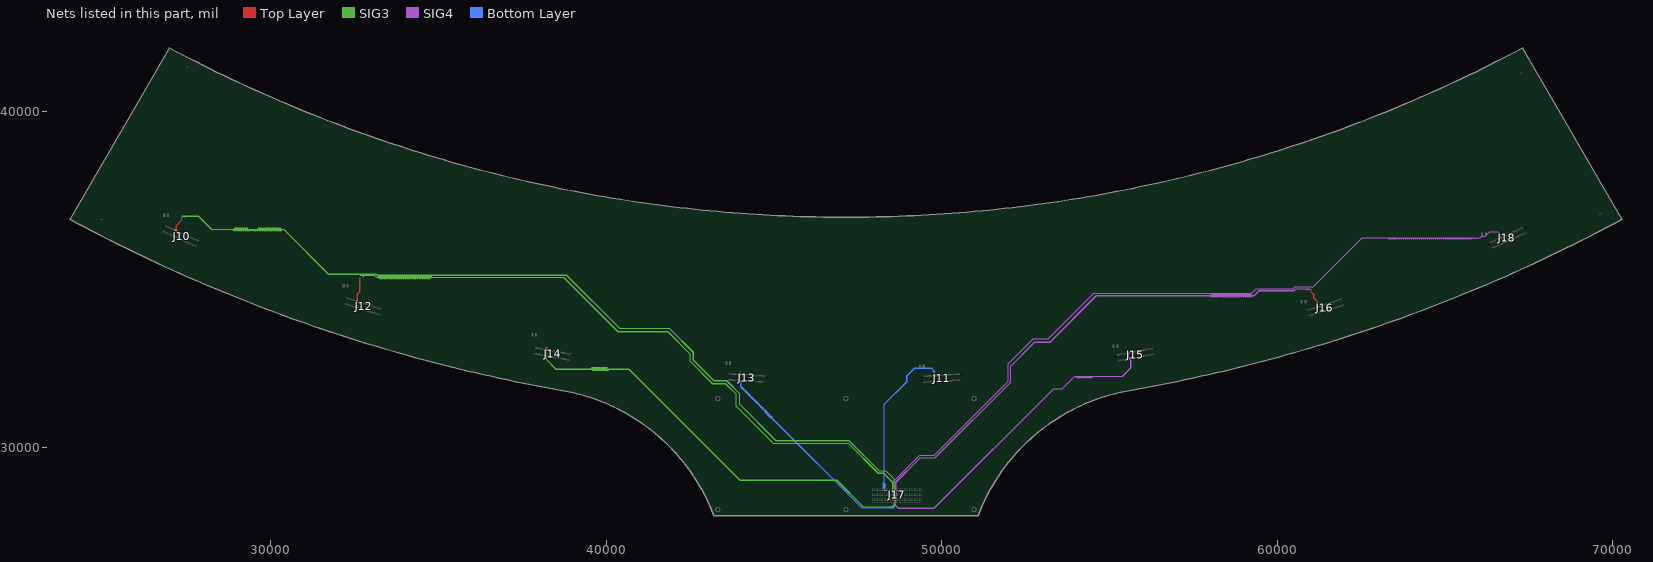
[diagram p0: the nets of this part, all layers, seen from the top]
# Altium PCB MISC86329.PcbDoc (part 6 of 11)
Units mil, origin at the board's own origin, x right, y up, seen from the top; angles counter-clockwise.
Board outline 46247.15 x 13937.21 mil, 6 copper layers (Top Layer, GND2, SIG3, SIG4, POWER5, Bottom Layer); 17 components, 210 nets, 908 pads, 1109 vias.

## Via types
v1: diameter 24, hole 12, Top Layer to Bottom Layer, 684 vias
v2: diameter 18, hole 9, Top Layer to Bottom Layer, 425 vias

## Nets (pads, with @x,y where several pads share a name; then routed paths per layer and width w, separated by ;. In a path a pad name is that pad's centre, name@x,y a point inside that pad or via, vN(x,y) a via of type N, cw(c..) or ccw(c..) an arc to the next point about the centre after c; other vN are vias at no path point) (continued)
DATAIN4N_CH0: J10.24 J17.G17 | length 28226.9
  Top Layer w5: J10.24@27193.09,36458.02 27193.09,36485.62 27204,36496.53 27204,36609 27363,36768 27363,36860.5 v2(27369.5,36867) ; v2(48564.09,28692.61) J17.G17@48587.89,28668.8
  SIG3 w5: v2(27369.5,36867) 27363,36873.5 27363,36882.86 27377.14,36897 27429,36897 27434,36892 27434,36882.36 27439,36877.36 27449,36877.36 27454,36882.36 27454,36892 27459,36897 27844,36897 27926,36815 ; 27925.93,36814.93 28242.86,36498 28888.68,36498 28894.5,36492.18 28894.5,36470.06 28906.18,36458.39 28927.82,36458.39 28939.5,36470.06 28939.5,36531.79 28945.32,36537.61 28958.68,36537.61 28964.5,36531.79 28964.5,36470.06 28976.18,36458.39 28997.82,36458.39 29009.5,36470.06 29009.5,36531.79 29015.32,36537.61 29028.68,36537.61 29034.5,36531.79 29034.5,36470.07 29046.18,36458.39 29067.82,36458.39 29079.5,36470.07 29079.5,36531.79 29085.32,36537.61 29098.68,36537.61 29104.5,36531.79 29104.5,36470.07 29116.18,36458.39 29137.82,36458.39 29149.5,36470.07 29149.5,36531.79 29155.32,36537.61 29168.68,36537.61 29174.5,36531.79 29174.5,36470.07 29186.18,36458.39 29207.82,36458.39 29219.5,36470.07 29219.5,36531.79 29225.32,36537.61 29238.68,36537.61 29244.5,36531.79 29244.5,36470.07 29256.18,36458.39 29277.82,36458.39 29289.5,36470.07 29289.5,36531.79 29295.32,36537.61 29308.68,36537.61 29314.5,36531.79 29314.5,36470.07 29326.18,36458.39 29347.82,36458.39 29359.5,36470.07 29359.5,36492.18 29365.32,36498 29378.68,36498 29384.5,36492.18 29384.5,36470.07 29396.18,36458.39 29417.82,36458.39 29429.5,36470.07 29429.5,36492.18 29435.32,36498 29448.68,36498 29454.5,36492.18 29454.5,36470.07 29466.18,36458.39 29487.82,36458.39 29499.5,36470.07 29499.5,36492.18 29505.32,36498 29518.68,36498 29524.5,36492.18 29524.5,36470.07 29536.18,36458.39 29557.82,36458.39 29569.5,36470.07 29569.5,36492.18 29575.32,36498 29588.68,36498 29594.5,36492.18 29594.5,36470.07 29606.18,36458.39 29627.82,36458.39 29639.5,36470.07 29639.5,36531.79 29645.32,36537.61 29658.68,36537.61 29664.5,36531.79 29664.5,36470.07 29676.18,36458.39 29697.82,36458.39 29709.5,36470.07 29709.5,36531.79 29715.32,36537.61 29728.68,36537.61 29734.5,36531.79 29734.5,36470.07 29746.18,36458.39 29767.82,36458.39 29779.5,36470.07 29779.5,36531.79 29785.32,36537.61 29798.68,36537.61 29804.5,36531.79 29804.5,36470.07 29816.18,36458.39 29837.82,36458.39 29849.5,36470.07 29849.5,36531.79 29855.32,36537.61 29868.68,36537.61 29874.5,36531.79 29874.5,36470.07 29886.18,36458.39 29907.82,36458.39 29919.5,36470.07 29919.5,36531.79 29925.32,36537.61 29938.68,36537.61 29944.5,36531.79 29944.5,36470.07 29956.18,36458.39 29977.82,36458.39 29989.5,36470.07 29989.5,36531.79 29995.32,36537.61 30008.68,36537.61 30014.5,36531.79 30014.5,36470.07 30026.18,36458.39 30047.82,36458.39 30059.5,36470.07 30059.5,36531.79 30065.32,36537.61 30078.68,36537.61 30084.5,36531.79 30084.5,36470.07 30096.18,36458.39 30117.82,36458.39 30129.5,36470.07 30129.5,36531.79 30135.32,36537.61 30148.68,36537.61 30154.5,36531.79 30154.5,36470.07 30166.18,36458.39 30187.82,36458.39 30199.5,36470.07 30199.5,36531.79 30205.32,36537.61 30218.68,36537.61 30224.5,36531.79 30224.5,36470.07 30236.18,36458.39 30257.82,36458.39 30269.5,36470.07 30269.5,36531.79 30275.32,36537.61 30288.68,36537.61 30294.5,36531.79 30294.5,36470.07 30306.18,36458.39 30327.82,36458.39 30339.5,36470.07 30339.5,36492.18 30345.32,36498 30391.86,36498 31719.86,35170 33145.86,35170 33173.86,35142 38814.86,35142 40405.86,33551 41879,33551 42599,32831 42599,32597.86 43201.86,31995 43588,31995 43977,31606 43977,31291.86 45058.86,30210 47233.86,30210 48140.86,29303 48332.09,29303 48584.09,29051 48584.09,28712.61 v2(48564.09,28692.61)
DATAIN4N_CH1: J12.24 J17.F17 | length 23094.6
  Top Layer w5: J12.24@32606.57,34348.01 32606.57,34368.43 32602,34373 32602,34580.86 32673,34651.86 32673,35083.5 v2(32679.5,35090) ; v2(48564.09,28642.61) J17.F17@48587.89,28618.8
  SIG3 w5: v2(32679.5,35090) 32673,35096.5 32673,35104.86 32696.14,35128 32721,35128 32733.5,35128 32752.25,35128 32758.5,35121.75 32758.5,35094.45 32764.75,35088.2 32777.25,35088.2 32783.5,35094.45 32783.5,35121.75 32789.75,35128 32953,35128 33094.86,35128 33152.86,35070 33203.82,35070 33215.5,35081.68 33215.5,35104.08 33221.32,35109.9 33234.68,35109.9 33240.5,35104.08 33240.5,35041.78 33252.18,35030.1 33273.82,35030.1 33285.5,35041.78 33285.5,35104.08 33291.32,35109.9 33304.68,35109.9 33310.5,35104.08 33310.5,35041.78 33322.18,35030.1 33343.82,35030.1 33355.5,35041.78 33355.5,35104.08 33361.32,35109.9 33374.68,35109.9 33380.5,35104.08 33380.5,35041.78 33392.18,35030.1 33413.82,35030.1 33425.5,35041.78 33425.5,35104.08 33431.32,35109.9 33444.68,35109.9 33450.5,35104.08 33450.5,35041.78 33462.18,35030.1 33483.82,35030.1 33495.5,35041.78 33495.5,35104.08 33501.32,35109.9 33514.68,35109.9 33520.5,35104.08 33520.5,35041.78 33532.18,35030.1 33553.82,35030.1 33565.5,35041.78 33565.5,35104.08 33571.32,35109.9 33584.68,35109.9 33590.5,35104.08 33590.5,35041.78 33602.18,35030.1 33623.82,35030.1 33635.5,35041.78 33635.5,35104.08 33641.32,35109.9 33654.68,35109.9 33660.5,35104.08 33660.5,35041.78 33672.18,35030.1 33693.82,35030.1 33705.5,35041.78 33705.5,35104.08 33711.32,35109.9 33724.68,35109.9 33730.5,35104.08 33730.5,35041.78 33742.18,35030.1 33763.82,35030.1 33775.5,35041.78 33775.5,35104.08 33781.32,35109.9 33794.68,35109.9 33800.5,35104.08 33800.5,35041.78 33812.18,35030.1 33833.82,35030.1 33845.5,35041.78 33845.5,35104.08 33851.32,35109.9 33864.68,35109.9 33870.5,35104.08 33870.5,35041.78 33882.18,35030.1 33903.82,35030.1 33915.5,35041.78 33915.5,35104.08 33921.32,35109.9 33934.68,35109.9 33940.5,35104.08 33940.5,35041.78 33952.18,35030.1 33973.82,35030.1 33985.5,35041.78 33985.5,35104.08 33991.32,35109.9 34004.68,35109.9 34010.5,35104.08 34010.5,35041.78 34022.18,35030.1 34043.82,35030.1 34055.5,35041.78 34055.5,35104.08 34061.32,35109.9 34074.68,35109.9 34080.5,35104.08 34080.5,35041.78 34092.18,35030.1 34113.82,35030.1 34125.5,35041.78 34125.5,35104.08 34131.32,35109.9 34144.68,35109.9 34150.5,35104.08 34150.5,35041.78 34162.18,35030.1 34183.82,35030.1 34195.5,35041.78 34195.5,35104.08 34201.32,35109.9 34214.68,35109.9 34220.5,35104.08 34220.5,35041.78 34232.18,35030.1 34253.82,35030.1 34265.5,35041.78 34265.5,35104.08 34271.32,35109.9 34284.68,35109.9 34290.5,35104.08 34290.5,35041.78 34302.18,35030.1 34323.82,35030.1 34335.5,35041.78 34335.5,35104.08 34341.32,35109.9 34354.68,35109.9 34360.5,35104.08 34360.5,35041.78 34372.18,35030.1 34393.82,35030.1 34405.5,35041.78 34405.5,35104.08 34411.32,35109.9 34424.68,35109.9 34430.5,35104.08 34430.5,35041.78 34442.18,35030.1 34463.82,35030.1 34475.5,35041.78 34475.5,35104.08 34481.32,35109.9 34494.68,35109.9 34500.5,35104.08 34500.5,35041.78 34512.18,35030.1 34533.82,35030.1 34545.5,35041.78 34545.5,35104.08 34551.32,35109.9 34564.68,35109.9 34570.5,35104.08 34570.5,35041.78 34582.18,35030.1 34603.82,35030.1 34615.5,35041.78 34615.5,35104.08 34621.32,35109.9 34634.68,35109.9 34640.5,35104.08 34640.5,35041.78 34652.18,35030.1 34673.82,35030.1 34685.5,35041.78 34685.5,35104.08 34691.32,35109.9 34704.68,35109.9 34710.5,35104.08 34710.5,35041.78 34722.18,35030.1 34743.82,35030.1 34755.5,35041.78 34755.5,35104.08 34761.32,35109.9 34774.68,35109.9 34780.5,35104.08 34780.5,35081.68 34792.18,35070 38727.86,35070 40348.86,33449 41834,33449 42502,32781 42502,32570.86 43163.86,31909 43546,31909 43873,31582 43873,31229.86 44976.86,30126 47211,30126 48101,29236 48254.86,29236 48535,28955.86 48535,28671.69 48554.66,28652.04 v2(48564.09,28642.61)
DATAIN4N_CH2: J14.24 J17.B17 | length 13805.5
  Top Layer w5: v2(38232.5,33011) 38226,33004.5 38226,32944 38236.84,32933.16 J14.24@38236.84,32913.47 ; v2(48564.09,28395) J17.B17@48587.89,28418.8
  SIG3 w5: v2@38230,33008 38225,33003 38225,32971.14 38239,32957.14 38239,32924.75 38245.25,32918.5 38250.95,32918.5 38257.2,32912.25 38257.2,32899.75 38250.95,32893.5 38245.25,32893.5 38239,32887.25 38239,32617 38507,32349 39566.68,32349 39572.5,32354.82 39572.5,32377.05 39584.18,32388.72 39605.82,32388.72 39617.5,32377.05 39617.5,32315.1 39623.32,32309.28 39636.68,32309.28 39642.5,32315.1 39642.5,32377.05 39654.18,32388.72 39675.82,32388.72 39687.5,32377.05 39687.5,32315.1 39693.32,32309.28 39706.68,32309.28 39712.5,32315.1 39712.5,32377.05 39724.18,32388.72 39745.82,32388.72 39757.5,32377.05 39757.5,32315.1 39763.32,32309.28 39776.68,32309.28 39782.5,32315.1 39782.5,32377.05 39794.18,32388.72 39815.82,32388.72 39827.5,32377.05 39827.5,32315.1 39833.32,32309.28 39846.68,32309.28 39852.5,32315.1 39852.5,32377.05 39864.18,32388.72 39885.82,32388.72 39897.5,32377.05 39897.5,32315.1 39903.32,32309.28 39916.68,32309.28 39922.5,32315.1 39922.5,32377.05 39934.18,32388.72 39955.82,32388.72 39967.5,32377.05 39967.5,32315.1 39973.32,32309.28 39986.68,32309.28 39992.5,32315.1 39992.5,32377.05 40004.18,32388.72 40025.82,32388.72 40037.5,32377.05 40037.5,32315.1 40043.32,32309.28 40056.68,32309.28 40062.5,32315.1 40062.5,32337.32 40074.18,32349 40681,32349 43989,29041 46869,29041 47670,28240 48527.09,28240 48584.09,28297 48584.09,28375 v2(48564.09,28395)
DATAIN4N_CH3: J13.24 J17.A17 | length 7743
  Top Layer w5: 43989.26,32238.5 43989.26,32215.72 43999.98,32205 J13.24@43999.98,32175.77 ; v2(48564.09,28345) J17.A17@48587.89,28368.8
  Bottom Layer w5: v2@43995,32244 43990,32239 43990,32203 43990,32196.75 43996.25,32190.5 44011.15,32190.5 44017.4,32184.25 44017.4,32171.75 44011.15,32165.5 43996.25,32165.5 43990,32159.25 43990,32116 43990,32003 44024,31969 44024,31807.14 44039.03,31792.12 44043.72,31792.12 44049.03,31797.42 44062.01,31797.42 44073.77,31785.65 44073.77,31772.67 44068.47,31767.37 44068.47,31762.67 44074.38,31756.76 44079.08,31756.76 44084.38,31762.06 44097.36,31762.06 44109.13,31750.3 44109.13,31737.32 44103.83,31732.01 44103.83,31727.32 44109.74,31721.41 44114.43,31721.41 44119.74,31726.71 44132.72,31726.71 44144.49,31714.94 44144.49,31701.96 44139.18,31696.66 44139.18,31691.96 44145.09,31686.05 44149.79,31686.05 44155.09,31691.35 44168.07,31691.35 44179.84,31679.59 44179.84,31666.6 44174.54,31661.3 44174.54,31656.6 44180.45,31650.69 44185.14,31650.69 44190.45,31656 44203.43,31656 44215.2,31644.23 44215.2,31631.25 44209.89,31625.95 44209.89,31621.25 44215.8,31615.34 44220.5,31615.34 44225.8,31620.64 44238.78,31620.64 44250.55,31608.88 44250.55,31595.89 44245.25,31590.59 44245.25,31585.89 44251.16,31579.98 44255.85,31579.98 44261.16,31585.29 44274.14,31585.29 44285.91,31573.52 44285.91,31560.54 44280.6,31555.24 44280.6,31550.54 44286.51,31544.63 44291.21,31544.63 44296.51,31549.93 44309.49,31549.93 44321.26,31538.16 44321.26,31525.18 44315.96,31519.88 44315.96,31515.18 44321.87,31509.27 44326.57,31509.27 44331.87,31514.58 44344.85,31514.58 44356.62,31502.81 44356.62,31489.83 44351.31,31484.52 44351.31,31479.83 44357.22,31473.92 44361.92,31473.92 44367.22,31479.22 44380.2,31479.22 44391.97,31467.45 44391.97,31454.47 44386.67,31449.17 44386.67,31444.47 44392.58,31438.56 44397.28,31438.56 44402.58,31443.87 44415.56,31443.87 44427.33,31432.1 44427.33,31419.12 44422.02,31413.81 44422.02,31409.12 44427.93,31403.21 44432.63,31403.21 44437.93,31408.51 44450.92,31408.51 44462.68,31396.74 44462.68,31383.76 44457.38,31378.46 44457.38,31373.76 44463.29,31367.85 44467.99,31367.85 44473.29,31373.16 44486.27,31373.16 44498.04,31361.39 44498.04,31348.41 44492.74,31343.1 44492.74,31338.41 44498.65,31332.5 44503.34,31332.5 44508.65,31337.8 44521.63,31337.8 44533.39,31326.03 44533.39,31313.05 44528.09,31307.75 44528.09,31303.05 44534,31297.14 44538.7,31297.14 44544,31302.44 44556.98,31302.44 44568.75,31290.68 44568.75,31277.7 44563.45,31272.39 44563.45,31267.7 44569.36,31261.79 44574.05,31261.79 44579.36,31267.09 44592.34,31267.09 44604.1,31255.32 44604.1,31242.34 44598.8,31237.04 44598.8,31232.34 44604.71,31226.43 44609.41,31226.43 44614.71,31231.73 44627.69,31231.73 44639.46,31219.97 44639.46,31206.99 44634.16,31201.68 44634.16,31196.99 44640.07,31191.08 44644.76,31191.08 44650.07,31196.38 44663.05,31196.38 44674.82,31184.61 44674.82,31171.63 44669.51,31166.33 44669.51,31161.63 44675.42,31155.72 44680.12,31155.72 44685.42,31161.02 44698.4,31161.02 44710.17,31149.26 44710.17,31136.27 44704.87,31130.97 44704.87,31126.27 44710.78,31120.36 44715.47,31120.36 44720.78,31125.67 44733.76,31125.67 44745.53,31113.9 44745.53,31100.92 44740.22,31095.62 44740.22,31090.92 44746.13,31085.01 44750.83,31085.01 44756.13,31090.31 44769.11,31090.31 44780.88,31078.54 44780.88,31065.56 44761.44,31046.12 44761.44,31041.42 44767.35,31035.51 44772.04,31035.51 44791.49,31054.96 44804.47,31054.96 44816.24,31043.19 44816.24,31030.21 44796.79,31010.76 44796.79,31006.07 44802.7,31000.16 44807.4,31000.16 44826.84,31019.6 44839.82,31019.6 44851.59,31007.83 44851.59,30994.85 44832.15,30975.41 44832.15,30970.71 44838.06,30964.8 44842.75,30964.8 44862.2,30984.25 44875.18,30984.25 44886.95,30972.48 44886.95,30959.5 44867.5,30940.05 44867.5,30935.36 44873.41,30929.45 44878.11,30929.45 44897.55,30948.89 44910.54,30948.89 44922.3,30937.12 44922.3,30924.14 44902.86,30904.7 44902.86,30900 44908.77,30894.09 44913.46,30894.09 44932.91,30913.54 44945.89,30913.54 44957.66,30901.77 44957.66,30888.79 44952.35,30883.48 44952.35,30878.79 47621.14,28210 48429.18,28210 48432.5,28213.32 48432.5,28220.82 48441.68,28230 48458.32,28230 48467.5,28220.82 48467.5,28213.32 48470.82,28210 48479.18,28210 48482.5,28213.32 48482.5,28220.82 48491.68,28230 48508.32,28230 48517.5,28220.82 48517.5,28213.32 48520.82,28210 48563,28210 48584.09,28231.09 48584.09,28243.18 48580.77,28246.5 48573.27,28246.5 48564.09,28255.68 48564.09,28272.32 48573.27,28281.5 48600.77,28281.5 48604.09,28284.82 48604.09,28293.18 48600.77,28296.5 48593.27,28296.5 48584.09,28305.68 48584.09,28325 v2(48564.09,28345)
  other v2: 43995.76,32245
DATAIN4N_CH4: J11.24 J17.H23 | length 5094.1
  Top Layer w5: v2(48264.09,28742.61) J17.H23@48287.89,28718.8 ; v2(49805.83,32210) 49799.33,32203.5 49799.33,32181.72 49810.05,32171 J11.24@49810.05,32145.93
  Bottom Layer w5: v2(48264.09,28742.61) 48284.09,28762.61 48284.09,28787.93 48281.02,28791 48263.02,28791 48254.09,28799.93 48254.09,28822.07 48263.02,28831 48311.02,28831 48314.09,28834.07 48314.09,28847.93 48311.02,28851 48263.02,28851 48254.09,28859.93 48254.09,28882.07 48263.02,28891 48311.02,28891 48314.09,28894.07 48314.09,28907.93 48311.02,28911 48263.02,28911 48254.09,28919.93 48254.09,28942.07 48263.02,28951 48281.02,28951 48284.09,28954.07 48284.09,31288.09 48960,31964 48960,32146.14 49192.86,32379 49685.14,32379 49726.07,32338.07 49763.32,32300.82 49799,32265.14 49799,32218 v2@49806,32211
DATAIN4N_CH5: J15.24 J17.C17 | length 10126.3
  Top Layer w5: v2(48564.09,28445) J17.C17@48587.89,28468.8 ; 55567,32889.5 55567,32863.46 55580.46,32850 J15.24@55580.46,32824.38
  SIG4 w5: v2(48564.09,28445) 48584.09,28425 48584.09,28314.77 48703.86,28195 49785.14,28195 53339.14,31749 53595.14,31749 53968.14,32122 54019.43,32122 54024,32117.43 54024,32093.53 54034.43,32083.1 54053.57,32083.1 54064,32093.53 54064,32117.43 54068.57,32122 54079.43,32122 54084,32117.43 54084,32093.53 54094.43,32083.1 54113.57,32083.1 54124,32093.53 54124,32117.43 54128.57,32122 54139.43,32122 54144,32117.43 54144,32093.53 54154.43,32083.1 54173.57,32083.1 54184,32093.53 54184,32117.43 54188.57,32122 54199.43,32122 54204,32117.43 54204,32093.53 54214.43,32083.1 54233.57,32083.1 54244,32093.53 54244,32117.43 54248.57,32122 54259.43,32122 54264,32117.43 54264,32093.53 54274.43,32083.1 54293.57,32083.1 54304,32093.53 54304,32117.43 54308.57,32122 54319.43,32122 54324,32117.43 54324,32093.53 54334.43,32083.1 54353.57,32083.1 54364,32093.53 54364,32117.43 54368.57,32122 54379.43,32122 54384,32117.43 54384,32093.53 54394.43,32083.1 54413.57,32083.1 54424,32093.53 54424,32117.43 54428.57,32122 54439.43,32122 54444,32117.43 54444,32093.53 54454.43,32083.1 54473.57,32083.1 54484,32093.53 54484,32117.43 54488.57,32122 55391.14,32122 55645,32375.86 55645,32608.14 55567,32686.14 55567,32789 55567,32807 55567,32837 55567,32852 55567,32862 55567,32880 ; 55567,32883 55567,32880 ; v2@55574,32897 55567,32890 55567,32880
  other v2: 55573.5,32896
DATAIN4N_CH6: J16.24 J17.D17 | length 18293.3
  Top Layer w5: v2(48564.09,28495) J17.D17@48587.89,28518.8 ; 61004,34691.5 61004,34645.14 61099,34550.14 61099,34458.14 61209,34348.14 61209,34217.17 J16.24@61225.17,34201
  SIG4 w5: v2(48564.09,28495) 48590.75,28495 48607.25,28511.5 48616.44,28511.5 48634,28529.06 48634,28976.14 49358.86,29701 49799,29701 52051,31953 52051,32430.14 52775.86,33155 53234,33155 54612,34533 57994.14,34533 58022.14,34505 58031.86,34505 58038,34511.14 58038,34552.57 58048.43,34563 58067.57,34563 58078,34552.57 58078,34507.57 58082.57,34503 58093.43,34503 58098,34507.57 58098,34552.57 58108.43,34563 58127.57,34563 58138,34552.57 58138,34507.57 58142.57,34503 58153.43,34503 58158,34507.57 58158,34552.57 58168.43,34563 58187.57,34563 58198,34552.57 58198,34507.57 58202.57,34503 58213.43,34503 58218,34507.57 58218,34552.57 58228.43,34563 58247.57,34563 58258,34552.57 58258,34507.57 58262.57,34503 58273.43,34503 58278,34507.57 58278,34552.57 58288.43,34563 58307.57,34563 58318,34552.57 58318,34507.57 58322.57,34503 58333.43,34503 58338,34507.57 58338,34552.57 58348.43,34563 58367.57,34563 58378,34552.57 58378,34507.57 58382.57,34503 58393.43,34503 58398,34507.57 58398,34552.57 58408.43,34563 58427.57,34563 58438,34552.57 58438,34507.57 58442.57,34503 58453.43,34503 58458,34507.57 58458,34552.57 58468.43,34563 58487.57,34563 58498,34552.57 58498,34507.57 58502.57,34503 58513.43,34503 58518,34507.57 58518,34552.57 58528.43,34563 58547.57,34563 58558,34552.57 58558,34507.57 58562.57,34503 58573.43,34503 58578,34507.57 58578,34552.57 58588.43,34563 58607.57,34563 58618,34552.57 58618,34507.57 58622.57,34503 58633.43,34503 58638,34507.57 58638,34552.57 58648.43,34563 58667.57,34563 58678,34552.57 58678,34507.57 58682.57,34503 58693.43,34503 58698,34507.57 58698,34552.57 58708.43,34563 58727.57,34563 58738,34552.57 58738,34507.57 58742.57,34503 58753.43,34503 58758,34507.57 58758,34552.57 58768.43,34563 58787.57,34563 58798,34552.57 58798,34507.57 58802.57,34503 58813.43,34503 58818,34507.57 58818,34552.57 58828.43,34563 58847.57,34563 58858,34552.57 58858,34507.57 58862.57,34503 58873.43,34503 58878,34507.57 58878,34552.57 58888.43,34563 58907.57,34563 58918,34552.57 58918,34507.57 58922.57,34503 58933.43,34503 58938,34507.57 58938,34552.57 58948.43,34563 58967.57,34563 58978,34552.57 58978,34507.57 58982.57,34503 58993.43,34503 58998,34507.57 58998,34552.57 59008.43,34563 59027.57,34563 59038,34552.57 59038,34507.57 59042.57,34503 59053.43,34503 59058,34507.57 59058,34552.57 59068.43,34563 59087.57,34563 59098,34552.57 59098,34507.57 59102.57,34503 59113.43,34503 59118,34507.57 59118,34552.57 59128.43,34563 59147.57,34563 59158,34552.57 59158,34507.57 59162.57,34503 59173.43,34503 59178,34507.57 59178,34552.57 59188.43,34563 59207.57,34563 59218,34552.57 59218,34507.57 59222.57,34503 59233.43,34503 59238,34507.57 59238,34522.57 59248.43,34533 59309,34533 59457,34681 60507,34681 60563,34737 60984.14,34737 61005,34716.14 61005,34709 ; 61005,34707 61005,34709 ; v2@61011,34698 61005,34704 61005,34709
  other v2: 61010.5,34698
DATAIN4N_CH7: J17.E17 J18.24 | length 23897.3
  Top Layer w5: v2(48564.09,28545) J17.E17@48587.89,28568.8 ; v2(66617.5,36388) 66611,36381.5 66611,36364.14 66641.37,36333.78 66641.37,36273.96 J18.24@66660.04,36255.28
  SIG4 w5: v2(48564.09,28545) 48584.09,28565 48584.09,29006.23 49344.86,29767 49774,29767 51979,31972 51979,32499.14 52725.86,33246 53173,33246 54524,34597 59234,34597 59371,34734 60469,34734 60531,34796 61078,34796 62537,36255 63316.57,36255 63327,36244.57 63327,36229.57 63331.57,36225 63342.43,36225 63347,36229.57 63347,36244.57 63357.43,36255 63376.57,36255 63387,36244.57 63387,36229.57 63391.57,36225 63402.43,36225 63407,36229.57 63407,36244.57 63417.43,36255 63436.57,36255 63447,36244.57 63447,36229.57 63451.57,36225 63462.43,36225 63467,36229.57 63467,36244.57 63477.43,36255 63496.57,36255 63507,36244.57 63507,36229.57 63511.57,36225 63522.43,36225 63527,36229.57 63527,36244.57 63537.43,36255 63556.57,36255 63567,36244.57 63567,36229.57 63571.57,36225 63582.43,36225 63587,36229.57 63587,36244.57 63597.43,36255 63616.57,36255 63627,36244.57 63627,36229.57 63631.57,36225 63642.43,36225 63647,36229.57 63647,36244.57 63657.43,36255 63676.57,36255 63687,36244.57 63687,36229.57 63691.57,36225 63702.43,36225 63707,36229.57 63707,36244.57 63717.43,36255 63736.57,36255 63747,36244.57 63747,36229.57 63751.57,36225 63762.43,36225 63767,36229.57 63767,36244.57 63777.43,36255 63796.57,36255 63807,36244.57 63807,36229.57 63811.57,36225 63822.43,36225 63827,36229.57 63827,36244.57 63837.43,36255 63856.57,36255 63867,36244.57 63867,36229.57 63871.57,36225 63882.43,36225 63887,36229.57 63887,36244.57 63897.43,36255 63916.57,36255 63927,36244.57 63927,36229.57 63931.57,36225 63942.43,36225 63947,36229.57 63947,36244.57 63957.43,36255 63976.57,36255 63987,36244.57 63987,36229.57 63991.57,36225 64002.43,36225 64007,36229.57 64007,36244.57 64017.43,36255 64036.57,36255 64047,36244.57 64047,36229.57 64051.57,36225 64062.43,36225 64067,36229.57 64067,36244.57 64077.43,36255 64096.57,36255 64107,36244.57 64107,36229.57 64111.57,36225 64122.43,36225 64127,36229.57 64127,36244.57 64137.43,36255 64156.57,36255 64167,36244.57 64167,36229.57 64171.57,36225 64182.43,36225 64187,36229.57 64187,36244.57 64197.43,36255 64216.57,36255 64227,36244.57 64227,36229.57 64231.57,36225 64242.43,36225 64247,36229.57 64247,36244.57 64257.43,36255 64276.57,36255 64287,36244.57 64287,36229.57 64291.57,36225 64302.43,36225 64307,36229.57 64307,36244.57 64317.43,36255 64336.57,36255 64347,36244.57 64347,36229.57 64351.57,36225 64362.43,36225 64367,36229.57 64367,36244.57 64377.43,36255 64396.57,36255 64407,36244.57 64407,36229.57 64411.57,36225 64422.43,36225 64427,36229.57 64427,36244.57 64437.43,36255 64456.57,36255 64467,36244.57 64467,36229.57 64471.57,36225 64482.43,36225 64487,36229.57 64487,36244.57 64497.43,36255 64516.57,36255 64527,36244.57 64527,36229.57 64531.57,36225 64542.43,36225 64547,36229.57 64547,36244.57 64557.43,36255 64576.57,36255 64587,36244.57 64587,36229.57 64591.57,36225 64602.43,36225 64607,36229.57 64607,36244.57 64617.43,36255 64636.57,36255 64647,36244.57 64647,36229.57 64651.57,36225 64662.43,36225 64667,36229.57 64667,36244.57 64677.43,36255 64696.57,36255 64707,36244.57 64707,36229.57 64711.57,36225 64722.43,36225 64727,36229.57 64727,36244.57 64737.43,36255 64756.57,36255 64767,36244.57 64767,36229.57 64771.57,36225 64782.43,36225 64787,36229.57 64787,36244.57 64797.43,36255 64816.57,36255 64827,36244.57 64827,36229.57 64831.57,36225 64842.43,36225 64847,36229.57 64847,36244.57 64857.43,36255 64876.57,36255 64887,36244.57 64887,36229.57 64891.57,36225 64902.43,36225 64907,36229.57 64907,36244.57 64917.43,36255 64936.57,36255 64947,36244.57 64947,36229.57 64951.57,36225 64962.43,36225 64967,36229.57 64967,36244.57 64977.43,36255 64996.57,36255 65007,36244.57 65007,36229.57 65011.57,36225 65022.43,36225 65027,36229.57 65027,36244.57 65037.43,36255 65056.57,36255 65067,36244.57 65067,36229.57 65071.57,36225 65082.43,36225 65087,36229.57 65087,36244.57 65097.43,36255 65116.57,36255 65127,36244.57 65127,36229.57 65131.57,36225 65142.43,36225 65147,36229.57 65147,36244.57 65157.43,36255 65176.57,36255 65187,36244.57 65187,36229.57 65191.57,36225 65202.43,36225 65207,36229.57 65207,36244.57 65217.43,36255 65236.57,36255 65247,36244.57 65247,36229.57 65251.57,36225 65262.43,36225 65267,36229.57 65267,36244.57 65277.43,36255 65296.57,36255 65307,36244.57 65307,36229.57 65311.57,36225 65322.43,36225 65327,36229.57 65327,36244.57 65337.43,36255 65356.57,36255 65367,36244.57 65367,36229.57 65371.57,36225 65382.43,36225 65387,36229.57 65387,36244.57 65397.43,36255 65416.57,36255 65427,36244.57 65427,36229.57 65431.57,36225 65442.43,36225 65447,36229.57 65447,36244.57 65457.43,36255 65476.57,36255 65487,36244.57 65487,36229.57 65491.57,36225 65502.43,36225 65507,36229.57 65507,36244.57 65517.43,36255 65536.57,36255 65547,36244.57 65547,36229.57 65551.57,36225 65562.43,36225 65567,36229.57 65567,36244.57 65577.43,36255 65596.57,36255 65607,36244.57 65607,36229.57 65611.57,36225 65622.43,36225 65627,36229.57 65627,36244.57 65637.43,36255 65656.57,36255 65667,36244.57 65667,36229.57 65671.57,36225 65682.43,36225 65687,36229.57 65687,36244.57 65697.43,36255 65716.57,36255 65727,36244.57 65727,36229.57 65731.57,36225 65742.43,36225 65747,36229.57 65747,36244.57 65757.43,36255 65776.57,36255 65787,36244.57 65787,36229.57 65791.57,36225 65802.43,36225 65807,36229.57 65807,36244.57 65817.43,36255 65862,36255 65880,36237 65955,36237 65973,36255 66054,36255 66098,36299 66200,36299 66333,36432 66587,36432 66610,36409 66610,36396 v2@66616,36390
DATAIN4P_CH0: J10.22 J17.G16 | length 28227.1
  Top Layer w5: J10.22@27164.45,36471.12 27194,36500.67 27194,36613.14 27353,36772.14 27353,36860.5 v2(27346.5,36867) ; v2(48614.09,28692.61) J17.G16@48637.89,28668.8
  SIG3 w5: v2(27346.5,36867) 27353,36873.5 27353,36887 27373,36907 27848.14,36907 27936,36819.14 27936,36819 28247,36508 28892.82,36508 28904.5,36496.32 28904.5,36474.21 28910.32,36468.39 28923.68,36468.39 28929.5,36474.21 28929.5,36535.94 28941.18,36547.61 28962.82,36547.61 28974.5,36535.94 28974.5,36474.21 28980.32,36468.39 28993.68,36468.39 28999.5,36474.21 28999.5,36535.93 29011.18,36547.61 29032.82,36547.61 29044.5,36535.93 29044.5,36474.21 29050.32,36468.39 29063.68,36468.39 29069.5,36474.21 29069.5,36535.93 29081.18,36547.61 29102.82,36547.61 29114.5,36535.93 29114.5,36474.21 29120.32,36468.39 29133.68,36468.39 29139.5,36474.21 29139.5,36535.93 29151.18,36547.61 29172.82,36547.61 29184.5,36535.93 29184.5,36474.21 29190.32,36468.39 29203.68,36468.39 29209.5,36474.21 29209.5,36535.93 29221.18,36547.61 29242.82,36547.61 29254.5,36535.93 29254.5,36474.21 29260.32,36468.39 29273.68,36468.39 29279.5,36474.21 29279.5,36535.93 29291.18,36547.61 29312.82,36547.61 29324.5,36535.93 29324.5,36474.21 29330.32,36468.39 29343.68,36468.39 29349.5,36474.21 29349.5,36496.32 29361.18,36508 29382.82,36508 29394.5,36496.32 29394.5,36474.21 29400.32,36468.39 29413.68,36468.39 29419.5,36474.21 29419.5,36496.32 29431.18,36508 29452.82,36508 29464.5,36496.32 29464.5,36474.21 29470.32,36468.39 29483.68,36468.39 29489.5,36474.21 29489.5,36496.32 29501.18,36508 29522.82,36508 29534.5,36496.32 29534.5,36474.21 29540.32,36468.39 29553.68,36468.39 29559.5,36474.21 29559.5,36496.32 29571.18,36508 29592.82,36508 29604.5,36496.32 29604.5,36474.21 29610.32,36468.39 29623.68,36468.39 29629.5,36474.21 29629.5,36535.93 29641.18,36547.61 29662.82,36547.61 29674.5,36535.93 29674.5,36474.21 29680.32,36468.39 29693.68,36468.39 29699.5,36474.21 29699.5,36535.93 29711.18,36547.61 29732.82,36547.61 29744.5,36535.93 29744.5,36474.21 29750.32,36468.39 29763.68,36468.39 29769.5,36474.21 29769.5,36535.93 29781.18,36547.61 29802.82,36547.61 29814.5,36535.93 29814.5,36474.21 29820.32,36468.39 29833.68,36468.39 29839.5,36474.21 29839.5,36535.93 29851.18,36547.61 29872.82,36547.61 29884.5,36535.93 29884.5,36474.21 29890.32,36468.39 29903.68,36468.39 29909.5,36474.21 29909.5,36535.93 29921.18,36547.61 29942.82,36547.61 29954.5,36535.93 29954.5,36474.21 29960.32,36468.39 29973.68,36468.39 29979.5,36474.21 29979.5,36535.93 29991.18,36547.61 30012.82,36547.61 30024.5,36535.93 30024.5,36474.21 30030.32,36468.39 30043.68,36468.39 30049.5,36474.21 30049.5,36535.93 30061.18,36547.61 30082.82,36547.61 30094.5,36535.93 30094.5,36474.21 30100.32,36468.39 30113.68,36468.39 30119.5,36474.21 30119.5,36535.93 30131.18,36547.61 30152.82,36547.61 30164.5,36535.93 30164.5,36474.21 30170.32,36468.39 30183.68,36468.39 30189.5,36474.21 30189.5,36535.93 30201.18,36547.61 30222.82,36547.61 30234.5,36535.93 30234.5,36474.21 30240.32,36468.39 30253.68,36468.39 30259.5,36474.21 30259.5,36535.93 30271.18,36547.61 30292.82,36547.61 30304.5,36535.93 30304.5,36474.21 30310.32,36468.39 30323.68,36468.39 30329.5,36474.21 30329.5,36496.32 30341.18,36508 30396,36508 31724,35180 33150,35180 33178,35152 38819,35152 40410,33561 41883.14,33561 42609,32835.14 42609,32602 43206,32005 43592.14,32005 43987,31610.14 43987,31296 45063,30220 47238,30220 48145,29313 48336.23,29313 48594.09,29055.14 48594.09,28712.61 v2(48614.09,28692.61)
DATAIN4P_CH1: J12.22 J17.F16 | length 23095.4
  Top Layer w5: J12.22@32576.55,34357.52 32576.55,34368.55 32592,34384 32592,34585 32663,34656 32663,35083.5 v2(32656.5,35090) ; v2(48614.09,28642.61) J17.F16@48637.89,28618.8
  SIG3 w5: v2(32656.5,35090) 32663,35096.5 32663,35109 32692,35138 32721,35138 32733.5,35138 32752.25,35138 32789.75,35138 32953,35138 33099,35138 33157,35080 33199.68,35080 33205.5,35085.82 33205.5,35108.22 33217.18,35119.9 33238.82,35119.9 33250.5,35108.22 33250.5,35045.92 33256.32,35040.1 33269.68,35040.1 33275.5,35045.92 33275.5,35108.22 33287.18,35119.9 33308.82,35119.9 33320.5,35108.22 33320.5,35045.92 33326.32,35040.1 33339.68,35040.1 33345.5,35045.92 33345.5,35108.22 33357.18,35119.9 33378.82,35119.9 33390.5,35108.22 33390.5,35045.92 33396.32,35040.1 33409.68,35040.1 33415.5,35045.92 33415.5,35108.22 33427.18,35119.9 33448.82,35119.9 33460.5,35108.22 33460.5,35045.92 33466.32,35040.1 33479.68,35040.1 33485.5,35045.92 33485.5,35108.22 33497.18,35119.9 33518.82,35119.9 33530.5,35108.22 33530.5,35045.92 33536.32,35040.1 33549.68,35040.1 33555.5,35045.92 33555.5,35108.22 33567.18,35119.9 33588.82,35119.9 33600.5,35108.22 33600.5,35045.92 33606.32,35040.1 33619.68,35040.1 33625.5,35045.92 33625.5,35108.22 33637.18,35119.9 33658.82,35119.9 33670.5,35108.22 33670.5,35045.92 33676.32,35040.1 33689.68,35040.1 33695.5,35045.92 33695.5,35108.22 33707.18,35119.9 33728.82,35119.9 33740.5,35108.22 33740.5,35045.92 33746.32,35040.1 33759.68,35040.1 33765.5,35045.92 33765.5,35108.22 33777.18,35119.9 33798.82,35119.9 33810.5,35108.22 33810.5,35045.92 33816.32,35040.1 33829.68,35040.1 33835.5,35045.92 33835.5,35108.22 33847.18,35119.9 33868.82,35119.9 33880.5,35108.22 33880.5,35045.92 33886.32,35040.1 33899.68,35040.1 33905.5,35045.92 33905.5,35108.22 33917.18,35119.9 33938.82,35119.9 33950.5,35108.22 33950.5,35045.92 33956.32,35040.1 33969.68,35040.1 33975.5,35045.92 33975.5,35108.22 33987.18,35119.9 34008.82,35119.9 34020.5,35108.22 34020.5,35045.92 34026.32,35040.1 34039.68,35040.1 34045.5,35045.92 34045.5,35108.22 34057.18,35119.9 34078.82,35119.9 34090.5,35108.22 34090.5,35045.92 34096.32,35040.1 34109.68,35040.1 34115.5,35045.92 34115.5,35108.22 34127.18,35119.9 34148.82,35119.9 34160.5,35108.22 34160.5,35045.92 34166.32,35040.1 34179.68,35040.1 34185.5,35045.92 34185.5,35108.22 34197.18,35119.9 34218.82,35119.9 34230.5,35108.22 34230.5,35045.92 34236.32,35040.1 34249.68,35040.1 34255.5,35045.92 34255.5,35108.22 34267.18,35119.9 34288.82,35119.9 34300.5,35108.22 34300.5,35045.92 34306.32,35040.1 34319.68,35040.1 34325.5,35045.92 34325.5,35108.22 34337.18,35119.9 34358.82,35119.9 34370.5,35108.22 34370.5,35045.92 34376.32,35040.1 34389.68,35040.1 34395.5,35045.92 34395.5,35108.22 34407.18,35119.9 34428.82,35119.9 34440.5,35108.22 34440.5,35045.92 34446.32,35040.1 34459.68,35040.1 34465.5,35045.92 34465.5,35108.22 34477.18,35119.9 34498.82,35119.9 34510.5,35108.22 34510.5,35045.92 34516.32,35040.1 34529.68,35040.1 34535.5,35045.92 34535.5,35108.22 34547.18,35119.9 34568.82,35119.9 34580.5,35108.22 34580.5,35045.92 34586.32,35040.1 34599.68,35040.1 34605.5,35045.92 34605.5,35108.22 34617.18,35119.9 34638.82,35119.9 34650.5,35108.22 34650.5,35045.92 34656.32,35040.1 34669.68,35040.1 34675.5,35045.92 34675.5,35108.22 34687.18,35119.9 34708.82,35119.9 34720.5,35108.22 34720.5,35045.92 34726.32,35040.1 34739.68,35040.1 34745.5,35045.92 34745.5,35108.22 34757.18,35119.9 34778.82,35119.9 34790.5,35108.22 34790.5,35085.82 34796.32,35080 38732,35080 40353,33459 41838.14,33459 42512,32785.14 42512,32575 43168,31919 43550.14,31919 43883,31586.14 43883,31234 44981,30136 47215.14,30136 48105.14,29246 48259,29246 48545,28960 48545,28675.83 48561.73,28659.11 48570.92,28659.11 48587.42,28642.61 v2(48614.09,28642.61)
DATAIN4P_CH2: J14.22 J17.B16 | length 13806.5
  Top Layer w5: J14.22@38205.88,32919.25 38205.88,32929.88 38216,32940 38216,33004.5 ; v2(48614.09,28395) J17.B16@48637.89,28418.8
  SIG3 w5: v2@38208,33012 38215,33005 38215,32967 38229,32953 38229,32924.75 38229,32612.86 38502.86,32339 39570.82,32339 39582.5,32350.68 39582.5,32372.9 39588.32,32378.72 39601.68,32378.72 39607.5,32372.9 39607.5,32310.95 39619.18,32299.28 39640.82,32299.28 39652.5,32310.95 39652.5,32372.9 39658.32,32378.72 39671.68,32378.72 39677.5,32372.9 39677.5,32310.95 39689.18,32299.28 39710.82,32299.28 39722.5,32310.95 39722.5,32372.9 39728.32,32378.72 39741.68,32378.72 39747.5,32372.9 39747.5,32310.95 39759.18,32299.28 39780.82,32299.28 39792.5,32310.95 39792.5,32372.9 39798.32,32378.72 39811.68,32378.72 39817.5,32372.9 39817.5,32310.95 39829.18,32299.28 39850.82,32299.28 39862.5,32310.95 39862.5,32372.9 39868.32,32378.72 39881.68,32378.72 39887.5,32372.9 39887.5,32310.95 39899.18,32299.28 39920.82,32299.28 39932.5,32310.95 39932.5,32372.9 39938.32,32378.72 39951.68,32378.72 39957.5,32372.9 39957.5,32310.95 39969.18,32299.28 39990.82,32299.28 40002.5,32310.95 40002.5,32372.9 40008.32,32378.72 40021.68,32378.72 40027.5,32372.9 40027.5,32310.95 40039.18,32299.28 40060.82,32299.28 40072.5,32310.95 40072.5,32333.18 40078.32,32339 40676.86,32339 43984.86,29031 46864.86,29031 47665.86,28230 48531.23,28230 48594.09,28292.86 48594.09,28375 v2(48614.09,28395)
  other v2: 38209.5,33011
DATAIN4P_CH3: J13.22 J17.A16 | length 7743.6
  Top Layer w5: J13.22@43968.54,32177.74 43968.54,32205 43979.26,32215.72 43979.26,32238.5 v2(43972.76,32245) ; v2(48614.09,28345) J17.A16@48637.89,28368.8
  Bottom Layer w5: v2@43974,32244 43974,32242 43980,32236 43980,32203 43980,32196.75 43980,32159.25 43980,32116 43980,31998.86 44014,31964.86 44014,31803 44034.88,31782.12 44047.86,31782.12 44053.17,31787.42 44057.86,31787.42 44063.77,31781.51 44063.77,31776.81 44058.47,31771.51 44058.47,31758.53 44070.24,31746.76 44083.22,31746.76 44088.52,31752.06 44093.22,31752.06 44099.13,31746.15 44099.13,31741.46 44093.83,31736.15 44093.83,31723.17 44105.59,31711.41 44118.58,31711.41 44123.88,31716.71 44128.58,31716.71 44134.49,31710.8 44134.49,31706.1 44129.18,31700.8 44129.18,31687.82 44140.95,31676.05 44153.93,31676.05 44159.23,31681.35 44163.93,31681.35 44169.84,31675.44 44169.84,31670.75 44164.54,31665.44 44164.54,31652.46 44176.31,31640.69 44189.29,31640.69 44194.59,31646 44199.29,31646 44205.2,31640.09 44205.2,31635.39 44199.89,31630.09 44199.89,31617.11 44211.66,31605.34 44224.64,31605.34 44229.94,31610.64 44234.64,31610.64 44240.55,31604.73 44240.55,31600.04 44235.25,31594.73 44235.25,31581.75 44247.02,31569.98 44260,31569.98 44265.3,31575.29 44270,31575.29 44275.91,31569.38 44275.91,31564.68 44270.6,31559.38 44270.6,31546.4 44282.37,31534.63 44295.35,31534.63 44300.66,31539.93 44305.35,31539.93 44311.26,31534.02 44311.26,31529.33 44305.96,31524.02 44305.96,31511.04 44317.73,31499.27 44330.71,31499.27 44336.01,31504.58 44340.71,31504.58 44346.62,31498.67 44346.62,31493.97 44341.31,31488.67 44341.31,31475.69 44353.08,31463.92 44366.06,31463.92 44371.37,31469.22 44376.06,31469.22 44381.97,31463.31 44381.97,31458.61 44376.67,31453.31 44376.67,31440.33 44388.44,31428.56 44401.42,31428.56 44406.72,31433.87 44411.42,31433.87 44417.33,31427.96 44417.33,31423.26 44412.02,31417.96 44412.02,31404.98 44423.79,31393.21 44436.77,31393.21 44442.08,31398.51 44446.77,31398.51 44452.68,31392.6 44452.68,31387.9 44447.38,31382.6 44447.38,31369.62 44459.15,31357.85 44472.13,31357.85 44477.43,31363.16 44482.13,31363.16 44488.04,31357.25 44488.04,31352.55 44482.74,31347.25 44482.74,31334.26 44494.5,31322.5 44507.48,31322.5 44512.79,31327.8 44517.48,31327.8 44523.39,31321.89 44523.39,31317.19 44518.09,31311.89 44518.09,31298.91 44529.86,31287.14 44542.84,31287.14 44548.14,31292.44 44552.84,31292.44 44558.75,31286.53 44558.75,31281.84 44553.45,31276.53 44553.45,31263.55 44565.21,31251.79 44578.19,31251.79 44583.5,31257.09 44588.19,31257.09 44594.1,31251.18 44594.1,31246.48 44588.8,31241.18 44588.8,31228.2 44600.57,31216.43 44613.55,31216.43 44618.85,31221.73 44623.55,31221.73 44629.46,31215.82 44629.46,31211.13 44624.16,31205.82 44624.16,31192.84 44635.92,31181.08 44648.91,31181.08 44654.21,31186.38 44658.91,31186.38 44664.82,31180.47 44664.82,31175.77 44659.51,31170.47 44659.51,31157.49 44671.28,31145.72 44684.26,31145.72 44689.56,31151.02 44694.26,31151.02 44700.17,31145.11 44700.17,31140.42 44694.87,31135.11 44694.87,31122.13 44706.64,31110.36 44719.62,31110.36 44724.92,31115.67 44729.62,31115.67 44735.53,31109.76 44735.53,31105.06 44730.22,31099.76 44730.22,31086.78 44741.99,31075.01 44754.97,31075.01 44760.27,31080.31 44764.97,31080.31 44770.88,31074.4 44770.88,31069.71 44751.44,31050.26 44751.44,31037.28 44763.2,31025.51 44776.18,31025.51 44795.63,31044.96 44800.33,31044.96 44806.24,31039.05 44806.24,31034.35 44786.79,31014.91 44786.79,31001.92 44798.56,30990.16 44811.54,30990.16 44830.99,31009.6 44835.68,31009.6 44841.59,31003.69 44841.59,30999 44822.15,30979.55 44822.15,30966.57 44833.91,30954.8 44846.9,30954.8 44866.34,30974.25 44871.04,30974.25 44876.95,30968.34 44876.95,30963.64 44857.5,30944.19 44857.5,30931.21 44869.27,30919.45 44882.25,30919.45 44901.7,30938.89 44906.39,30938.89 44912.3,30932.98 44912.3,30928.28 44892.86,30908.84 44892.86,30895.86 44904.63,30884.09 44917.61,30884.09 44937.05,30903.54 44941.75,30903.54 44947.66,30897.63 44947.66,30892.93 44942.35,30887.63 44942.35,30874.65 47617,28200 48433.32,28200 48442.5,28209.18 48442.5,28216.68 48445.82,28220 48454.18,28220 48457.5,28216.68 48457.5,28209.18 48466.68,28200 48483.32,28200 48492.5,28209.18 48492.5,28216.68 48495.82,28220 48504.18,28220 48507.5,28216.68 48507.5,28209.18 48516.68,28200 48567.14,28200 48594.09,28226.94 48594.09,28247.32 48584.91,28256.5 48577.41,28256.5 48574.09,28259.82 48574.09,28268.18 48577.41,28271.5 48604.91,28271.5 48614.09,28280.68 48614.09,28297.32 48604.91,28306.5 48597.41,28306.5 48594.09,28309.82 48594.09,28325 v2(48614.09,28345)
DATAIN4P_CH4: J11.22 J17.H22 | length 5093.8
  Top Layer w5: v2(48314.09,28742.61) J17.H22@48337.89,28718.8 ; J11.22@49778.61,32144.04 49778.61,32169 49789.33,32179.72 49789.33,32203.5
  Bottom Layer w5: v2(48314.09,28742.61) 48294.09,28762.61 48294.09,28792.07 48285.16,28801 48267.16,28801 48264.09,28804.07 48264.09,28817.93 48267.16,28821 48315.16,28821 48324.09,28829.93 48324.09,28852.07 48315.16,28861 48267.16,28861 48264.09,28864.07 48264.09,28877.93 48267.16,28881 48315.16,28881 48324.09,28889.93 48324.09,28912.07 48315.16,28921 48267.16,28921 48264.09,28924.07 48264.09,28937.93 48267.16,28941 48285.16,28941 48294.09,28949.93 48294.09,31283.94 48970,31959.86 48970,32142 49197,32369 49681,32369 49719,32331 49756.25,32293.75 49756.25,32286.68 49743.99,32274.42 49743.99,32267.35 49751.06,32260.28 49758.13,32260.28 49770.39,32272.54 49777.46,32272.54 49781,32269 49789,32261 49789,32218 v2@49784,32213
  other v2: 49782.83,32210
DATAIN4P_CH5: J15.22 J17.C16 | length 10125.7
  Top Layer w5: v2(48614.09,28445) J17.C16@48637.89,28468.8 ; J15.22@55549.48,32818.67 55549.48,32845 55557,32852.52 55557,32889.5
  SIG4 w5: v2(48614.09,28445) 48594.09,28425 48594.09,28318.91 48708,28205 49781,28205 53335,31759 53591,31759 53964,32132 54023.57,32132 54034,32121.57 54034,32097.68 54038.57,32093.1 54049.43,32093.1 54054,32097.68 54054,32121.57 54064.43,32132 54083.57,32132 54094,32121.57 54094,32097.68 54098.57,32093.1 54109.43,32093.1 54114,32097.68 54114,32121.57 54124.43,32132 54143.57,32132 54154,32121.57 54154,32097.68 54158.57,32093.1 54169.43,32093.1 54174,32097.68 54174,32121.57 54184.43,32132 54203.57,32132 54214,32121.57 54214,32097.68 54218.57,32093.1 54229.43,32093.1 54234,32097.68 54234,32121.57 54244.43,32132 54263.57,32132 54274,32121.57 54274,32097.68 54278.57,32093.1 54289.43,32093.1 54294,32097.68 54294,32121.57 54304.43,32132 54323.57,32132 54334,32121.57 54334,32097.68 54338.57,32093.1 54349.43,32093.1 54354,32097.68 54354,32121.57 54364.43,32132 54383.57,32132 54394,32121.57 54394,32097.68 54398.57,32093.1 54409.43,32093.1 54414,32097.68 54414,32121.57 54424.43,32132 54443.57,32132 54454,32121.57 54454,32097.68 54458.57,32093.1 54469.43,32093.1 54474,32097.68 54474,32121.57 54484.43,32132 55387,32132 55635,32380 55635,32604 55557,32682 55557,32789 55557,32807 55552,32812 55539.33,32812 55534.33,32817 55534.33,32827 55539.33,32832 55552,32832 55557,32837 55557,32852 55557,32862 55557,32880 55557,32893 v2@55553,32897
  other v2: 55550.5,32896
DATAIN4P_CH6: J16.22 J17.D16 | length 18292.4
  Top Layer w5: v2(48614.09,28495) J17.D16@48637.89,28518.8 ; v2(60987.5,34698) 60994,34691.5 60994,34641 61089,34546 61089,34454 61199,34344 61199,34215 61195.12,34211.12 J16.22@61195.12,34191.57
  SIG4 w5: v2(48614.09,28495) 48644,28524.91 48644,28972 49363,29691 49803.14,29691 52061,31948.86 52061,32426 52780,33145 53238.14,33145 54616.14,34523 57990,34523 58018,34495 58036,34495 58048,34507 58048,34548.43 58052.57,34553 58063.43,34553 58068,34548.43 58068,34503.43 58078.43,34493 58097.57,34493 58108,34503.43 58108,34548.43 58112.57,34553 58123.43,34553 58128,34548.43 58128,34503.43 58138.43,34493 58157.57,34493 58168,34503.43 58168,34548.43 58172.57,34553 58183.43,34553 58188,34548.43 58188,34503.43 58198.43,34493 58217.57,34493 58228,34503.43 58228,34548.43 58232.57,34553 58243.43,34553 58248,34548.43 58248,34503.43 58258.43,34493 58277.57,34493 58288,34503.43 58288,34548.43 58292.57,34553 58303.43,34553 58308,34548.43 58308,34503.43 58318.43,34493 58337.57,34493 58348,34503.43 58348,34548.43 58352.57,34553 58363.43,34553 58368,34548.43 58368,34503.43 58378.43,34493 58397.57,34493 58408,34503.43 58408,34548.43 58412.57,34553 58423.43,34553 58428,34548.43 58428,34503.43 58438.43,34493 58457.57,34493 58468,34503.43 58468,34548.43 58472.57,34553 58483.43,34553 58488,34548.43 58488,34503.43 58498.43,34493 58517.57,34493 58528,34503.43 58528,34548.43 58532.57,34553 58543.43,34553 58548,34548.43 58548,34503.43 58558.43,34493 58577.57,34493 58588,34503.43 58588,34548.43 58592.57,34553 58603.43,34553 58608,34548.43 58608,34503.43 58618.43,34493 58637.57,34493 58648,34503.43 58648,34548.43 58652.57,34553 58663.43,34553 58668,34548.43 58668,34503.43 58678.43,34493 58697.57,34493 58708,34503.43 58708,34548.43 58712.57,34553 58723.43,34553 58728,34548.43 58728,34503.43 58738.43,34493 58757.57,34493 58768,34503.43 58768,34548.43 58772.57,34553 58783.43,34553 58788,34548.43 58788,34503.43 58798.43,34493 58817.57,34493 58828,34503.43 58828,34548.43 58832.57,34553 58843.43,34553 58848,34548.43 58848,34503.43 58858.43,34493 58877.57,34493 58888,34503.43 58888,34548.43 58892.57,34553 58903.43,34553 58908,34548.43 58908,34503.43 58918.43,34493 58937.57,34493 58948,34503.43 58948,34548.43 58952.57,34553 58963.43,34553 58968,34548.43 58968,34503.43 58978.43,34493 58997.57,34493 59008,34503.43 59008,34548.43 59012.57,34553 59023.43,34553 59028,34548.43 59028,34503.43 59038.43,34493 59057.57,34493 59068,34503.43 59068,34548.43 59072.57,34553 59083.43,34553 59088,34548.43 59088,34503.43 59098.43,34493 59117.57,34493 59128,34503.43 59128,34548.43 59132.57,34553 59143.43,34553 59148,34548.43 59148,34503.43 59158.43,34493 59177.57,34493 59188,34503.43 59188,34548.43 59192.57,34553 59203.43,34553 59208,34548.43 59208,34503.43 59218.43,34493 59237.57,34493 59248,34503.43 59248,34518.43 59252.57,34523 59313.14,34523 59461.14,34671 60511.14,34671 60567.14,34727 60864,34727 60869,34722 60869,34711.07 60874,34706.07 60884,34706.07 60889,34711.07 60889,34722 60894,34727 60904,34727 60909,34722 60909,34711.07 60914,34706.07 60924,34706.07 60929,34711.07 60929,34722 60934,34727 60980,34727 60995,34712 60995,34707 60989,34701 v2@60988,34701